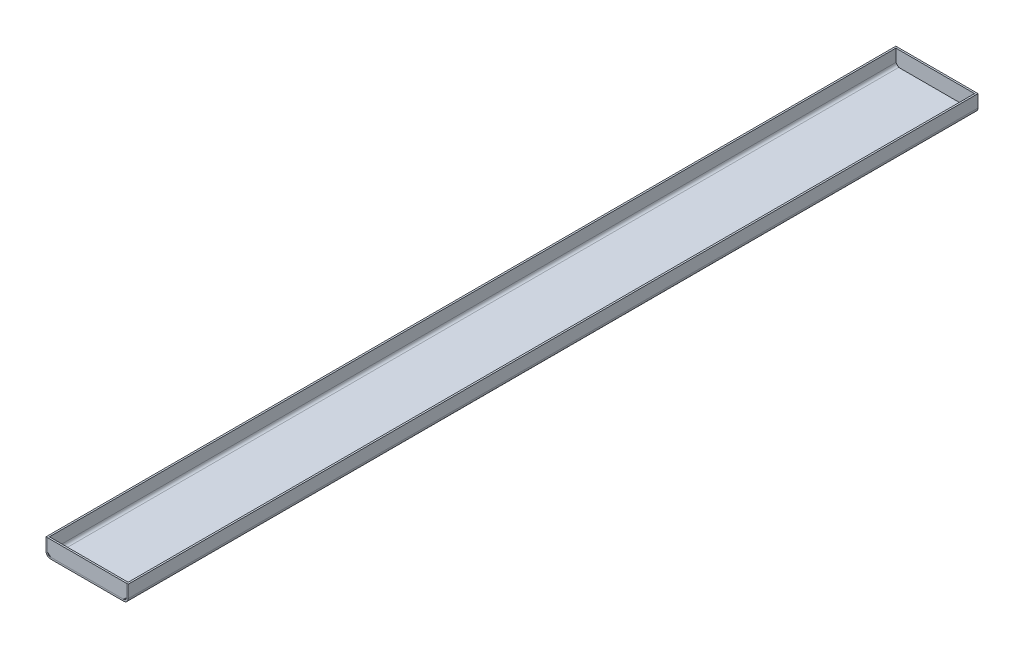
from build123d import *

# Parameters (mm, degrees)
BOSS_EXTRUDE1_DEPTH = 1500
BOSS_EXTRUDE2_DEPTH = 3
BOSS_EXTRUDE3_DEPTH = 3


with BuildPart() as part:
    # Sketch1 → Boss-Extrude1 (new body)
    with BuildSketch(Plane.XY):
        with BuildLine():
            Line((0, 0), (0, -22))
            ThreePointArc((0, -22), (2.343145751, -27.656854249), (8, -30))
            Line((8, -30), (137, -30))
            ThreePointArc((137, -30), (142.656854249, -27.656854249), (145, -22))
            Line((145, -22), (145, 0))
            Line((145, 0), (142, 0))
            Line((142, 0), (142, -22))
            ThreePointArc((142, -22), (140.535533906, -25.535533906), (137, -27))
            Line((137, -27), (8, -27))
            ThreePointArc((8, -27), (4.464466094, -25.535533906), (3, -22))
            Line((3, -22), (3, 0))
            Line((3, 0), (0, 0))
        make_face()
    extrude(amount=BOSS_EXTRUDE1_DEPTH)


with BuildPart() as body_2:
    # Sketch3 → Boss-Extrude2 (new body)
    with BuildSketch(Plane.XY.offset(1500)):
        Polygon((3, 0), (142, 0), (142, -22), (137, -27), (8, -27), (3, -22), align=None)
    extrude(amount=-BOSS_EXTRUDE2_DEPTH)


with BuildPart() as body_3:
    # Sketch4 → Boss-Extrude3 (new body)
    with BuildSketch(Plane(origin=(0, 0, 0), x_dir=(-1, 0, 0), z_dir=(0, 0, -1))):
        Polygon((-142, 0), (-3, 0), (-3, -22), (-8, -27), (-137, -27), (-142, -22), align=None)
    extrude(amount=-BOSS_EXTRUDE3_DEPTH)


solid = Compound([part.part, body_2.part, body_3.part])
